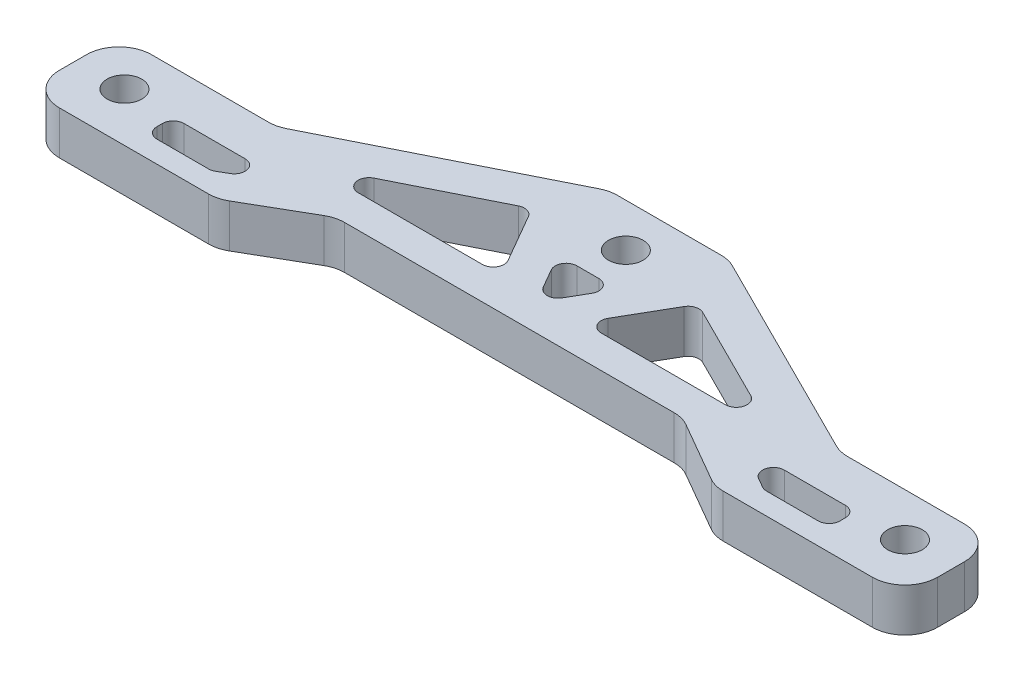
SolidWorks part; units mm, degrees
material "Thornel Mat VMA"
ref_plane "Front Plane" through (0, 0, 0) normal (0, 0, 1) x (1, 0, 0)
ref_plane "Top Plane" through (0, 0, 0) normal (0, 1, 0) x (1, 0, 0)
ref_plane "Right Plane" through (0, 0, 0) normal (1, 0, 0) x (0, 0, -1)
sketch "Sketch1" plane through (0, 0, 0) normal (0, 1, 0) x (1, 0, 0)
  line L0 (-36, 0) -> (36, 0) construction
  line L1 (0, 10.25) -> (0, 0) construction
  line L2 (-40.5, -4.5) -> (-22.9282, -4.5)
  line L3 (40.5, -4.5) -> (40.5, 4)
  line L4 (40.5, 4) -> (26, 4)
  line L6 (5.5, 14.25) -> (-5.5, 14.25)
  line L7 (-40.5, -4.5) -> (-40.5, 4)
  line L8 (-40.5, 4) -> (-26, 4)
  line L10 (-22.9282, -4.5) -> (-16, -0.5)
  line L11 (-16, -0.5) -> (16, -0.5)
  line L12 (16, -0.5) -> (22.9282, -4.5)
  line L13 (22.9282, -4.5) -> (40.5, -4.5)
  line L14 (-26, 4) -> (-5.5, 14.25)
  line L15 (26, 4) -> (5.5, 14.25)
  circle A0 centre (-36, 0) radius 1.6
  circle A1 centre (36, 0) radius 1.6
  circle A2 centre (0, 10.25) radius 1.6
  dimension "D1" = 10.25
  dimension "D2" = 3.2
  dimension "D3" = 72
  dimension "D4" = 4
  dimension "D5" = 4.5
  dimension "D6" = 4.5
  dimension "D7" = 10
  dimension "D8" = 150
  dimension "D9" = 0.5
  dimension "D10" = 32
  dimension "D11" = 4
  dimension "D12" = 11
extrude "Boss-Extrude1" add sketch "Sketch1" along normal blind 4
sketch "Sketch2" plane through (0, 4, 0) normal (0, 1, 0) x (1, 0, 0)
  line L0 (-36, 0) -> (0, 10.25) construction
  line L1 (0, 10.25) -> (36, 0) construction
  line L2 (-7.6552, 9.2593) -> (-21.1738, 2.5)
  line L3 (-21.1738, 2.5) -> (-3.7528, 2.5)
  line L4 (-3.7528, 2.5) -> (-7.6552, 9.2593)
  line L5 (-2.7424, 6.75) -> (0, 2)
  line L6 (-2.7424, 6.75) -> (2.7424, 6.75)
  line L7 (2.7424, 6.75) -> (0, 2)
  line L8 (0, 10.25) -> (0, 0) construction
  line L9 (21.1738, 2.5) -> (3.7528, 2.5)
  line L10 (7.6552, 9.2593) -> (21.1738, 2.5)
  line L11 (3.7528, 2.5) -> (7.6552, 9.2593)
  line L12 (-5.5, 14.25) -> (-26, 4) construction
  line L13 (-16, -0.5) -> (16, -0.5) construction
  line L14 (-31.5, 0) -> (-21.134, 0)
  line L15 (-21.134, 0) -> (-25.4641, -2.5)
  line L16 (-25.4641, -2.5) -> (-31.5, -2.5)
  line L17 (-31.5, -2.5) -> (-31.5, 0)
  line L18 (25.4641, -2.5) -> (31.5, -2.5)
  line L19 (21.134, 0) -> (25.4641, -2.5)
  line L20 (31.5, 0) -> (21.134, 0)
  line L21 (31.5, -2.5) -> (31.5, 0)
  line L22 (-40.5, -4.5) -> (-22.9282, -4.5) construction
  line L23 (-22.9282, -4.5) -> (-16, -0.5) construction
  dimension "D1" = 3.5
  dimension "D2" = 3
  dimension "D3" = 3.5
  dimension "D4" = 2.5
  dimension "D5" = 3
  dimension "D6" = 60
  dimension "D7" = 2.5
  dimension "D8" = 2
  dimension "D9" = 4.5
  dimension "D10" = 3
extrude "Cut-Extrude1" cut sketch "Sketch2" against normal through all
fillet "R1 cutout fillet" radius 1 17 edges at (21.1738, 2, -2.5) (3.7528, 2, -2.5) (7.6552, 2, -9.2593) (2.7424, 2, -6.75) (0, 2, -2) (-2.7424, 2, -6.75) (-3.7528, 2, -2.5) (-21.1738, 2, -2.5) (-7.6552, 2, -9.2593) (21.134, 2, 0) (31.5, 2, 2.5) (25.4641, 2, 2.5) (31.5, 2, 0) (-31.5, 2, 2.5) (-21.134, 2, 0) (-25.4641, 2, 2.5) (-31.5, 2, 0)
fillet "R3 outer edge fillet" radius 3 12 edges at (40.5, 2, -4) (40.5, 2, 4.5) (22.9282, 2, 4.5) (16, 2, 0.5) (-16, 2, 0.5) (-22.9282, 2, 4.5) (-40.5, 2, -4) (-26, 2, -4) (-5.5, 2, -14.25) (5.5, 2, -14.25) (26, 2, -4) (-40.5, 2, 4.5)
